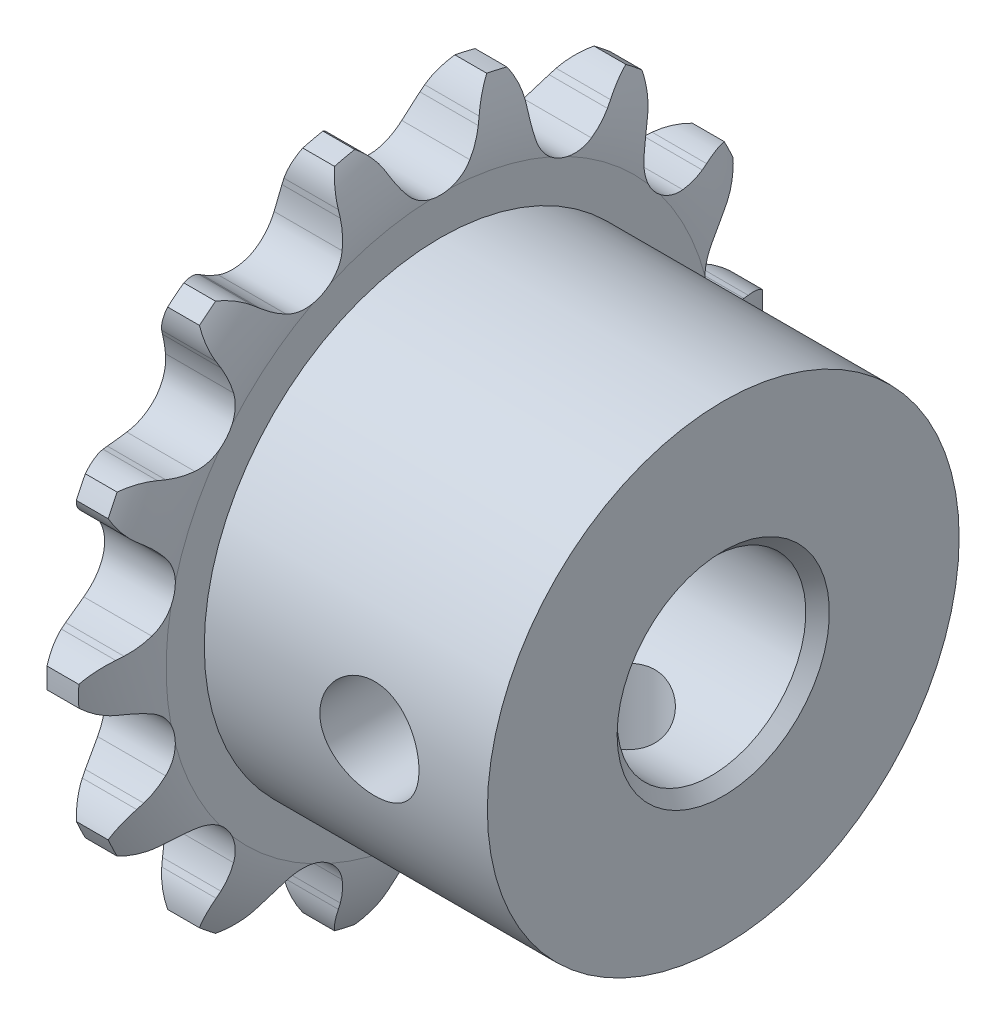
from build123d import *

# Parameters (mm, degrees)
EXTRUDECUTONE_DEPTH = 2.537198082
PATTERNONE_COUNT    = 14
SKETCH3_W           = 2.1
SKETCH3_H           = 14.227384256
CIRPATTERN1_COUNT   = 2
CIRPATTERN1_ANGLE   = 90
CHAMFER1_SIZE       = 0.5


with BuildPart() as part:
    # Sketch1 → Revolve 2 (revolve)
    with BuildSketch(Plane.XY, mode=Mode.PRIVATE) as revolve_2_sk:
        with BuildLine():
            Line((-1.5, 4), (-1.5, 9))
            Line((-1.5, 9), (-1.5, 11.616996164))
            ThreePointArc((-1.5, 11.616996164), (-1.259882344, 13.107928471), (-0.6745, 14.5))
            Line((-0.6745, 14.5), (0.6745, 14.5))
            ThreePointArc((0.6745, 14.5), (1.259882344, 13.107928471), (1.5, 11.616996164))
            Line((1.5, 11.616996164), (1.5, 10))
            Line((1.5, 10), (13.5, 10))
            Line((13.5, 10), (13.5, 4))
            Line((13.5, 4), (-1.5, 4))
        make_face()
    revolve(revolve_2_sk.sketch.rotate(Axis((-4, 0, 0), (1, 0, 0)), 90), axis=Axis((-4, 0, 0), (1, 0, 0)))

    # Sketch2 → ExtrudeCutOne (cut, symmetric)
    with BuildSketch(Plane(origin=(0, 0, 0), x_dir=(0, 0, -1), z_dir=(1, 0, 0))):
        with BuildLine():
            Line((1.877033772, 13.04944298), (1.99623343, 13.294673565))
            ThreePointArc((1.99623343, 13.294673565), (2.33688783, 13.81304378), (2.798488381, 14.227384256))
            ThreePointArc((2.798488381, 14.227384256), (0, 14.5), (-2.798488381, 14.227384256))
            ThreePointArc((-2.798488381, 14.227384256), (-2.33688783, 13.81304378), (-1.99623343, 13.294673565))
            Line((-1.99623343, 13.294673565), (-1.877033772, 13.04944298))
            ThreePointArc((-1.877033772, 13.04944298), (-1.622555123, 12.596822066), (-1.315936822, 12.177763249))
            ThreePointArc((-1.315936822, 12.177763249), (0, 11.558746164), (1.315936822, 12.177763249))
            ThreePointArc((1.315936822, 12.177763249), (1.622555123, 12.596822066), (1.877033772, 13.04944298))
        make_face()
    extrudecutone = extrude(amount=EXTRUDECUTONE_DEPTH, both=True, mode=Mode.SUBTRACT)

    # PatternOne: ExtrudeCutOne ×14 about axis
    patternone_axis = Axis((0, 0, 0), (1, 0, 0))
    for i in range(1, PATTERNONE_COUNT):
        add(extrudecutone.rotate(patternone_axis, i * 360 / PATTERNONE_COUNT), mode=Mode.SUBTRACT)

    # Sketch3 → M5 Tapped Hole1 (revolve, cut)
    with BuildSketch(Plane.YZ.offset(8.5)):
        with Locations((1.05, 7.113692128)):
            Rectangle(SKETCH3_W, SKETCH3_H)
    m5_tapped_hole1 = revolve(axis=Axis((8.5, 0, -6.35), (0, 0, 1)), mode=Mode.SUBTRACT)

    # CirPattern1: M5 Tapped Hole1 ×2 about axis
    cirpattern1_axis = Axis((-4, 0, 0), (1, 0, 0))
    for i in range(1, CIRPATTERN1_COUNT):
        add(m5_tapped_hole1.rotate(cirpattern1_axis, i * CIRPATTERN1_ANGLE / (CIRPATTERN1_COUNT - 1)), mode=Mode.SUBTRACT)

    # Chamfer1
    chamfer1_edges = [part.edges().sort_by_distance(p)[0] for p in [
        (13.5, 0, -4),
        (-1.5, 0, -4),
    ]]
    chamfer(chamfer1_edges, length=CHAMFER1_SIZE)


solid = part.part
